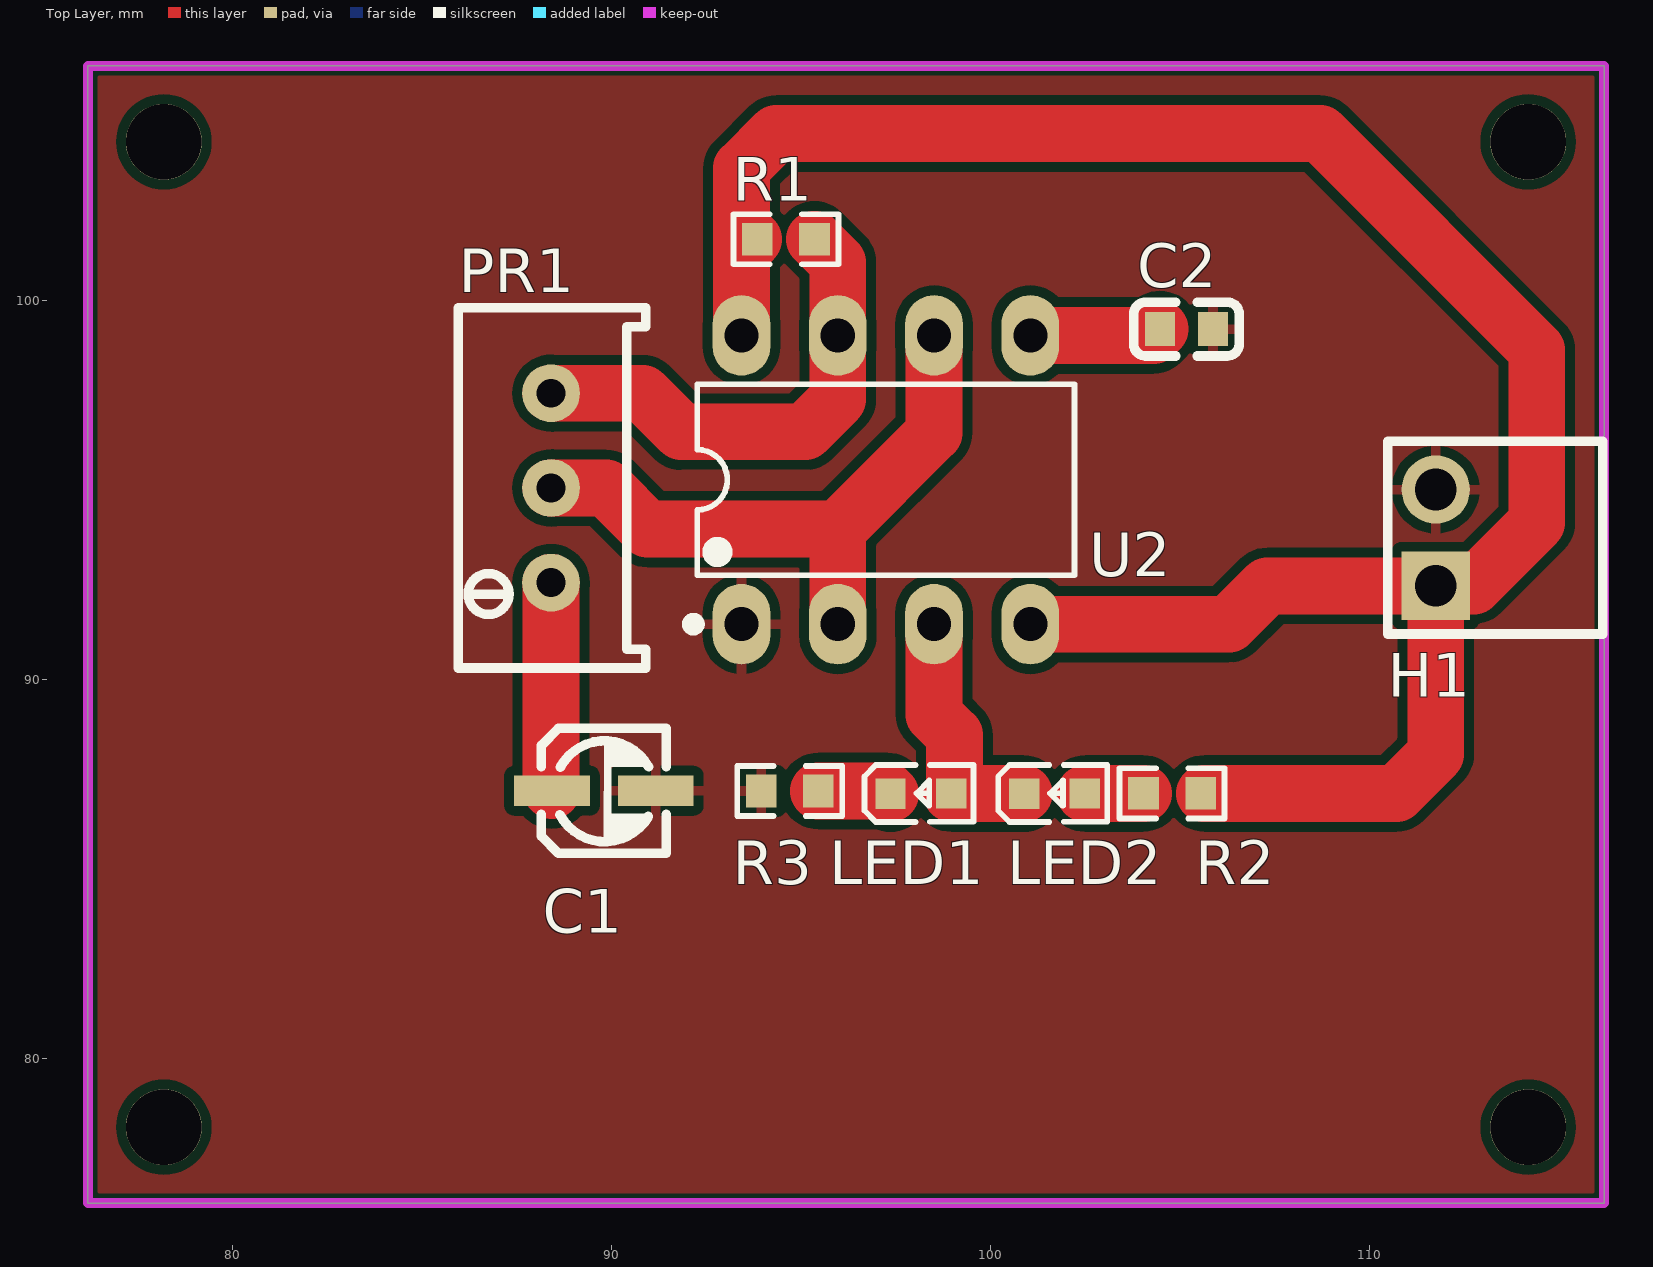
[diagram p0: Top Layer view]
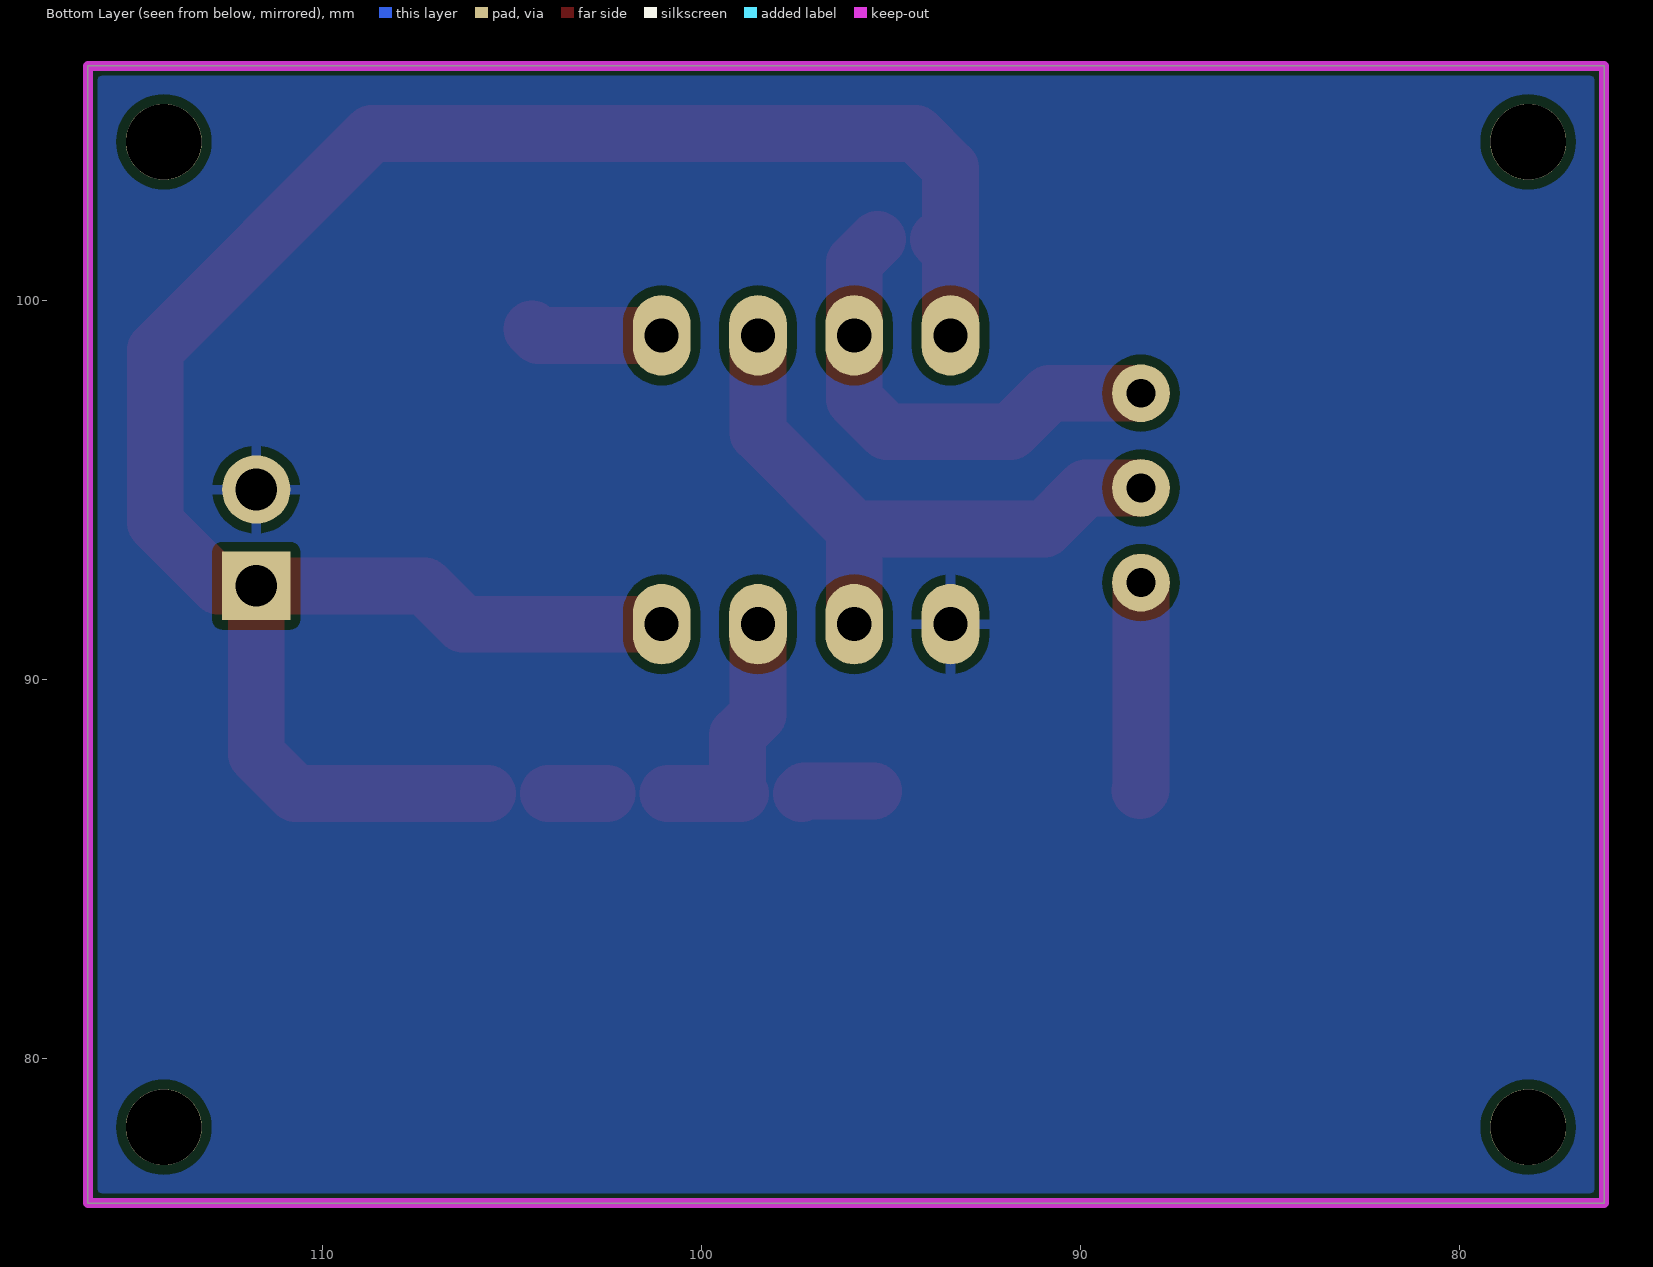
[diagram p1: Bottom Layer view, seen from below]
# Altium PCB MISC51886.pcbdoc
Units mm, origin at the board's own origin, x right, y up, seen from the top; angles counter-clockwise.
Board outline 40 x 30 mm, 2 copper layers (Top Layer, Bottom Layer), stack 1.58 mm thick; 10 components, 9 nets, 31 pads, 0 vias.

## Layer stack, top to bottom
Top Solder Mask Layer: solder mask 0.01, Dk 3.3
Top Layer: signal copper 0.035
Dielectric1: surface 1.51, FR4, Dk 4.5
Bottom Layer: signal copper 0.035
Bottom Solder Mask Layer: solder mask 0.01, Dk 3.3

## Board outline
76.2,106.2 76.2,76.2 116.2,76.2 116.2,106.2

## Design rules (kind name [scope] priority, off if disabled: settings)
BoardOutlineClearance copperThickness2oz_1 [All] p2 off: genericclearance=0.203 ignorepadtopadclearanceinfootprint=FALSE except(0: Arc-SplitContinuation Track-SplitContinuation SMDPad-SplitContinuation THPad-SplitContinuation Via-SplitContinuation Fill-SplitContinuation Region-SplitContinuation Poly-SplitContinuation Text-SplitContinuation Hole-SplitContinuation; 0.152: Arc-CutoutEdge SMDPad-CutoutEdge THPad-CutoutEdge Via-CutoutEdge Fill-CutoutEdge Region-CutoutEdge Text-CutoutEdge; 0.176: Hole-OutlineEdge Hole-CutoutEdge; 0.254: Poly-OutlineEdge Poly-CutoutEdge; 0.3: Arc-OutlineEdge Track-OutlineEdge SMDPad-OutlineEdge THPad-OutlineEdge Via-OutlineEdge Fill-OutlineEdge Region-OutlineEdge Text-OutlineEdge Track-CutoutEdge)
BoardOutlineClearance copperThickness1oz_1 [All] p4: genericclearance=0.102 ignorepadtopadclearanceinfootprint=FALSE except(0: Arc-SplitContinuation Track-SplitContinuation SMDPad-SplitContinuation THPad-SplitContinuation Via-SplitContinuation Fill-SplitContinuation Region-SplitContinuation Poly-SplitContinuation Text-SplitContinuation Hole-SplitContinuation; 0.152: SMDPad-CutoutEdge THPad-CutoutEdge Via-CutoutEdge Fill-CutoutEdge Region-CutoutEdge Text-CutoutEdge; 0.176: Hole-OutlineEdge Hole-CutoutEdge; 0.254: Poly-OutlineEdge Poly-CutoutEdge; 0.3: Arc-OutlineEdge Track-OutlineEdge SMDPad-OutlineEdge THPad-OutlineEdge Via-OutlineEdge Fill-OutlineEdge Region-OutlineEdge Text-OutlineEdge Arc-CutoutEdge Track-CutoutEdge)
Clearance copperThickness2oz [All] p1 off: gap=0.203 ignorepadtopadclearanceinfootprint=FALSE except(0.152: SMDPad-Track SMDPad-SMDPad THPad-Track SMDPad-THPad THPad-THPad Track-Via SMDPad-Via THPad-Via Via-Via Fill-Track Region-Track Fill-SMDPad Region-SMDPad Fill-THPad Region-THPad Fill-Via Region-Via Fill-Fill Fill-Region Region-Region Arc-Track Arc-SMDPad Arc-THPad Arc-Via Fill-Arc Region-Arc Arc-Arc Text-Track SMDPad-Text Text-THPad Text-Via Fill-Text Region-Text Arc-Text Text-Text; 0.176: Hole-Track Hole-SMDPad Hole-THPad Hole-Via Fill-Hole Region-Hole Hole-Arc Hole-Text; 0.254: Poly-Track Poly-SMDPad Poly-THPad Poly-Via Poly-Fill Poly-Region Poly-Poly Poly-Arc Poly-Text Poly-Hole)
Clearance copperThickness1oz [All] p3: gap=0.102 ignorepadtopadclearanceinfootprint=FALSE except(0.152: SMDPad-Track SMDPad-SMDPad THPad-Track SMDPad-THPad THPad-THPad Track-Via SMDPad-Via THPad-Via Via-Via Fill-Track Region-Track Fill-SMDPad Region-SMDPad Fill-THPad Region-THPad Fill-Via Region-Via Fill-Fill Fill-Region Region-Region Arc-Track Arc-SMDPad Arc-THPad Arc-Via Fill-Arc Region-Arc Arc-Arc Text-Track SMDPad-Text Text-THPad Text-Via Fill-Text Region-Text Arc-Text Text-Text; 0.176: Hole-Track Hole-SMDPad Hole-THPad Hole-Via Fill-Hole Region-Hole Hole-Arc Hole-Text; 0.254: Poly-Track Poly-SMDPad Poly-THPad Poly-Via Poly-Fill Poly-Region Poly-Poly Poly-Arc Poly-Text Poly-Hole)
Creepage creepage [All] p1: checkdistance=0 ignoreinternallayers=TRUE applytopolygonpour=TRUE
DiffPairsRouting differentialPair [All] p1: maxlimit=0.152 minlimit=0.152 mostfreqgap=0.152 toplayer_minwidth=0.127 toplayer_prefwidth=0.254 toplayer_maxwidth=2.54 toplayer_mingap=0.152 toplayer_prefgap=0.152 toplayer_maxgap=0.152 bottomlayer_minwidth=0.127 bottomlayer_prefwidth=0.254 bottomlayer_maxwidth=2.54 bottomlayer_mingap=0.152 bottomlayer_prefgap=0.152 bottomlayer_maxgap=0.152 maxuncoupledlength=0.254
HoleToHoleClearance otherClearance [All] p1: gap=0.3 allowstackedmicrovias=TRUE
Length netLength [All] p1: minlimit=0 maxlimit=0
MatchedLengths netLengthTolerance [All] p1: tolerance=25.4
PasteMaskExpansion pasteMaskExpansion [All] p1: expansion=0
PlaneConnect innerPlane [All] p1: planeconnectstyle=Relief reliefexpansion=0.508 reliefentries=4 reliefconductorwidth=0.254 reliefairgap=0.254
PolygonConnect copperRegion [(InNet('GND'))] p1: connectstyle=Relief reliefconductorwidth=0.254 reliefentries=4 polygonreliefangle="90 Angle" airgapwidth=0.254 via.connectstyle=Relief via.reliefconductorwidth=0.254 via.reliefentries=4 via.polygonreliefangle="90 Angle" via.airgapwidth=0.254
RoutingVias viaSize [All] p1: holewidth=0.305 width=0.61 viastyle="Through Hole" minholewidth=0.3 minwidth=0.5 maxholewidth=6.3 maxwidth=10
SolderMaskExpansion solderMaskExpansion [IsVia] p1: expansion=-25.4 istentingtop=TRUE
SolderMaskExpansion solderMaskExpansion [All] p2: expansion=0.051 istentingtop=FALSE
Width copperThickness2oz_2 [All] p1 off: maxlimit=2.54 minlimit=0.203 preferedwidth=0.254
Width copperThickness1oz_2 [All] p2: maxlimit=2.54 minlimit=0.127 preferedwidth=0.254

## Components (designator, comment, footprint, x,y, rotation, side; value= is the part's Value field where it differs from the comment)
C1 "10uF" C_Ele_SMD_3x5.4mm 89.816,87.066 r180 top
C2 "103" C0603 105.183,99.258 r180 top
H1 "" HDR-TH_2P-P2.54-V-M-1 111.76,93.754 r90 top
LED1 "" LED_0603 98.226,87.008 r0 top
LED2 "" LED_0603 101.754,87.008 r0 top
PR1 "100kΩ" R_3296 88.292,95.067 r90 top
R1 "4.7K" R0603 94.615,101.628 r180 top
R2 "1K" R0603 104.802,87.008 r0 top
R3 "100" R0603 94.713,87.072 r0 top
U2 "NE555" DIP-8_L9.8-W6.4-P2.54-LS7.6-BL 97.253,95.282 r0 top

## Footprints (in the part's own frame and the unit in brackets; to place one, negate y for a bottom-side part, rotate by r counter-clockwise, add the part's x,y. Pads: shape width x height; smd on the part's side, far side on the other; paste and mask are expansions set on the pad)
C0603 [mm]
  rect 0.8x0.9 smd: 1(-0.7,0) 2(0.7,0)
  silkscreen extent -1.39,-0.71 1.39,0.71
C_Ele_SMD_3x5.4mm [mil]
  rect 78.7x31.5 smd paste+0 mask+2: 1(54.1,-0.55) 2(-53.7,-0.55)
  silkscreen extent -65,-65 65,65
DIP-8_L9.8-W6.4-P2.54-LS7.6-BL [mm]
  oval 1.524x2.125 hole 0.9 paste+0 mask+0.051: 1(-3.81,-3.81) 2(-1.27,-3.81) 3(1.27,-3.81) 4(3.81,-3.81) 5(3.81,3.81) 6(1.27,3.81) 7(-1.27,3.81) 8(-3.81,3.81)
  silkscreen extent -5.23,-3.96 4.98,2.52
HDR-TH_2P-P2.54-V-M-1 [mm]
  rect 1.8x1.8 hole 1.1: 1(-1.27,0)
  round 1.8 hole 1.1: 2(1.27,0)
  silkscreen extent -2.54,-4.41 2.54,1.27
LED_0603 [mil]
  rect 31.5x31.5 smd paste+0 mask+2: 1(-33.5,-0.4) 2(29.5,-0.2)
  silkscreen extent -61,-30 53,30
R0603 [mm]
  rect 0.806x0.864 smd paste-100 mask+0.051: 1(-0.753,0) 2(0.753,0)
  silkscreen extent -1.39,-0.66 1.39,0.66
R_3296 [mil]
  round 60 hole 30 paste+0 mask+2: 1(-98.4,-5) 2(0,-5) 3(98.4,-5)
  silkscreen extent -187,-103 187,92

## Free pads (board coordinates)
  round 2 hole 2: 1(78.2,78.2) 1(78.2,104.2) 1(114.2,78.2) 1(114.2,104.2)

## Nets (pads, with @x,y where several pads share a name; then routed paths per layer and width w, separated by ;. In a path a pad name is that pad's centre, name@x,y a point inside that pad or via, vN(x,y) a via of type N, cw(c..) or ccw(c..) an arc to the next point about the centre after c; other vN are vias at no path point)
$1N13: PR1.3 R1.1 U2.7 | length 12.8
  Top Layer w1.5: PR1.3 90.836,97.567 91.854,96.548 95.123,96.548 95.983,97.408 U2.7 95.983,101.013 R1.1
$1N14: PR1.2 U2.2 U2.6 | length 16.7
  Top Layer w1.5: PR1.2 89.873,95.067 90.961,93.979 95.983,93.979 ; U2.2 95.983,93.979 ; U2.6 98.523,96.519 95.983,93.979
$1N15: C2.2 U2.5 | length 3.5
  Top Layer w1.5: U2.5 104.317,99.092 C2.2
$1N16: C1.1 PR1.1 | length 5.5
  Top Layer w1.5: PR1.1 88.419,87.103 C1.1
$1N18: LED1.2 LED2.1 U2.3 | length 6.6
  Top Layer w1.5: U2.3 98.523,89.084 99.06,88.547 LED1.2@99.06,87.003 ; LED1.2 LED1.2@99.06,87.003 ; LED2.1@100.901,86.998 100.896,87.003 LED1.2@99.06,87.003
$1N19: LED2.2 R2.1 | length 1.5
  Top Layer w1.5: LED2.2 102.509,87.008 R2.1
$1N20: LED1.1 R3.2 | length 1.9
  Top Layer w1.5: R3.2 97.3,87.072 LED1.1@97.374,86.998
GND: C1.2 C2.1 H1.2 R3.1 U2.1
VCC: H1.1 R1.2 R2.2 U2.4 U2.8 | length 58.6
  Top Layer w1.5: U2.8 93.443,101.305 ; R1.2@93.766,101.628 93.443,101.305 ; U2.4 106.303,91.472 107.315,92.484 H1.1 ; R2.2@105.651,87.008 110.729,87.008 111.76,88.039 H1.1 ; 93.443,101.305 93.443,103.504 94.361,104.422 108.712,104.422 114.427,98.707 114.427,94.149 112.762,92.484 H1.1

## Polygon pours and split planes (outlines as drawn)
GND on Top Layer (solid, remove dead copper, pour order 0): 76.2,106.2 76.2,76.2 116.2,76.2 116.2,106.2
GND on Bottom Layer (solid, remove dead copper, pour order 2): 76.2,106.2 76.2,76.2 116.2,76.2 116.2,106.2

## Keep-outs
Board Outline Layer:
  the board outline again, w0.254